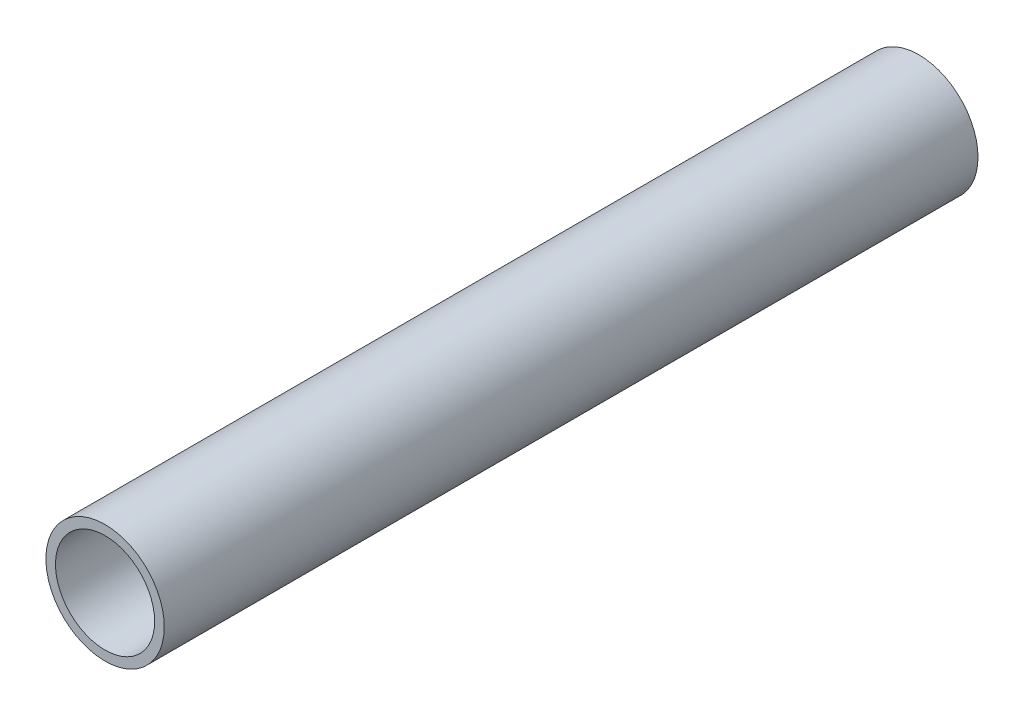
from build123d import *

# Parameters (mm, degrees)
SKETCH1_R           = 40
BOSS_EXTRUDE1_DEPTH = 550
SKETCH2_R           = 33.5
CUT_EXTRUDE1_DEPTH  = 90


with BuildPart() as part:
    # Sketch1 → Boss-Extrude1 (new body)
    with BuildSketch(Plane.XY):
        Circle(SKETCH1_R)
    extrude(amount=BOSS_EXTRUDE1_DEPTH)

    # Sketch2 → Cut-Extrude1 (cut)
    with BuildSketch(Plane.XY.offset(550)):
        Circle(SKETCH2_R)
    extrude(amount=-CUT_EXTRUDE1_DEPTH, mode=Mode.SUBTRACT)


solid = part.part
